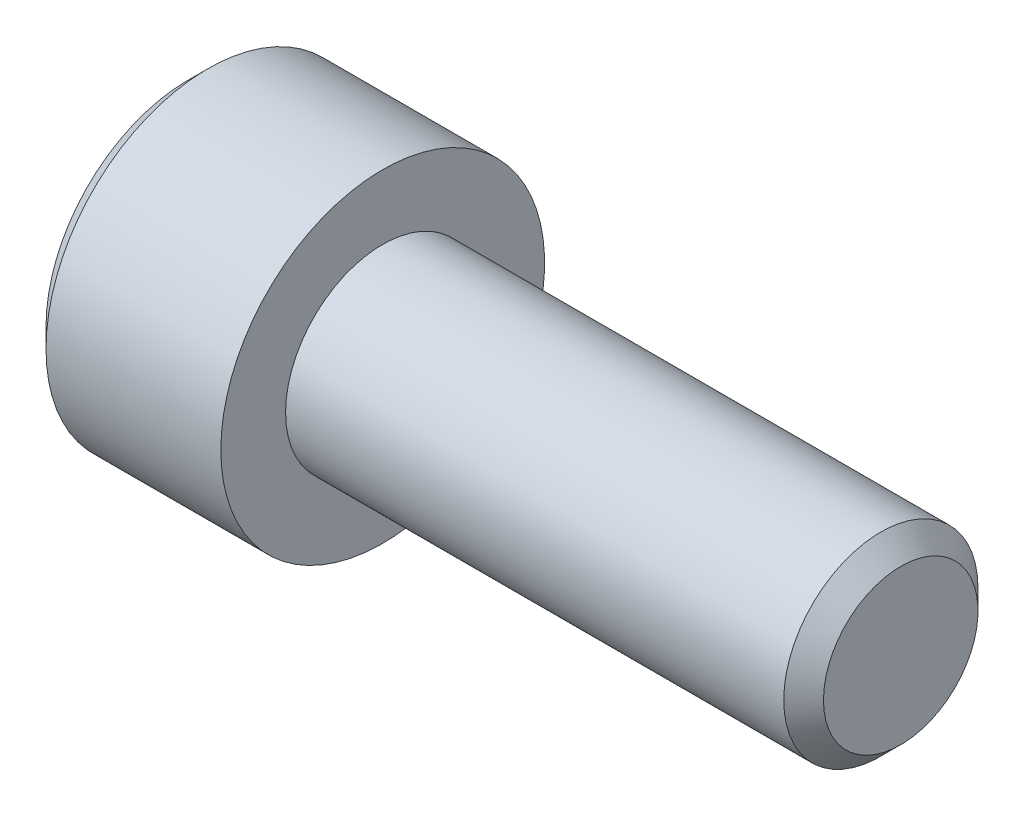
from build123d import *

# Parameters (mm, degrees)
CUT_EXTRUDE_1_DEPTH = 3


with BuildPart() as part:
    # 草图1 → 旋转1 (revolve)
    with BuildSketch(Plane.XY, mode=Mode.PRIVATE) as revolve_1_sk:
        Polygon((-6, 0), (-6, 4.4), (-5.4, 5), (0, 5), (0, 3), (15.3865, 3), (16, 2.3865), (16, 0), align=None)
    revolve(revolve_1_sk.sketch.rotate(Axis((16, 0, 0), (-1, 0, 0)), 270), axis=Axis((16, 0, 0), (-1, 0, 0)))

    # 草图2 → 切除-旋转1 (revolve, cut)
    with BuildSketch(Plane.XY, mode=Mode.PRIVATE) as cut_revolve_1_sk:
        Polygon((-6, 0), (-6, 2.5), (-3, 2.5), (-2.330127019, 0), align=None)
    revolve(cut_revolve_1_sk.sketch.rotate(Axis((-2.330127019, 0, 0), (-1, 0, 0)), 270), axis=Axis((-2.330127019, 0, 0), (-1, 0, 0)), mode=Mode.SUBTRACT)

    # 草图3 → 切除-拉伸1 (cut)
    with BuildSketch(Plane(origin=(-6, 0, 0), x_dir=(0, 0, -1), z_dir=(1, 0, 0))):
        Polygon((-2.5, 1.443375673), (-2.5, -1.443375673), (0, -2.886751346), (2.5, -1.443375673), (2.5, 1.443375673), (0, 2.886751346), align=None)
    extrude(amount=CUT_EXTRUDE_1_DEPTH, mode=Mode.SUBTRACT)


solid = part.part
